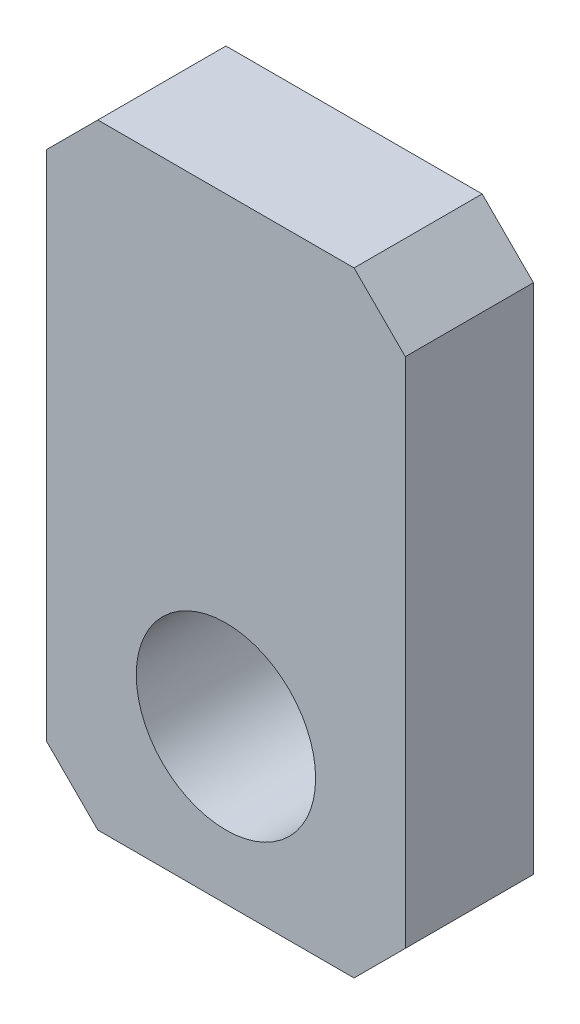
SolidWorks part; units mm, degrees
ref_plane "Front Plane" through (0, 0, 0) normal (0, 0, 1) x (1, 0, 0)
ref_plane "Top Plane" through (0, 0, 0) normal (0, 1, 0) x (1, 0, 0)
ref_plane "Right Plane" through (0, 0, 0) normal (1, 0, 0) x (0, 0, -1)
sketch "Sketch1" plane through (0, 0, 0) normal (0, 0, 1) x (1, 0, 0)
  line L1 (-3.5, 6) -> (3.5, 6)
  line L2 (-3.5, 6) -> (-3.5, -6)
  line L3 (-3.5, -6) -> (3.5, -6)
  line L4 (3.5, 6) -> (3.5, -6)
  line L5 (-3.5, 6) -> (3.5, -6) construction
  line L6 (-3.5, -6) -> (3.5, 6) construction
  point P0 (0, 0)
  dimension "D1" = 7
  dimension "D2" = 12
extrude "Boss-Extrude1" add sketch "Sketch1" along normal mid plane 2.5
hole_wizard "Ø3.5 (3.5) Diameter Hole1" positions "Sketch5" profile "Sketch4" hole size "Ø3.5" standard "Gb" end condition through all
sketch "Sketch5" plane through (0, 0, 1.25) normal (0, 0, 1) x (1, 0, 0)
  line L0 (-3.5, -6) -> (3.5, -6) construction
  point P0 (0, -3)
  dimension "D1" = 3
sketch "Sketch4" plane through (0, -3, 1.25) normal (1, 0, 0) x (0, -1, 0)
  line L0 (0, 0) -> (0, 2.5)
  line L1 (0, 2.5) -> (1.75, 2.5)
  line L2 (1.75, 2.5) -> (1.75, 0)
  line L5 (1.75, 0) -> (0, 0)
  line L11 (0, -6.35) -> (0, 107.95) construction
  dimension "通孔孔直径" = 3.5
  dimension "通孔孔深度" = 2.5
chamfer "Chamfer1" distance 1 angle 45 4 edges at (-3.5, -6, 0) (3.5, -6, 0) (-3.5, 6, 0) (3.5, 6, 0)
